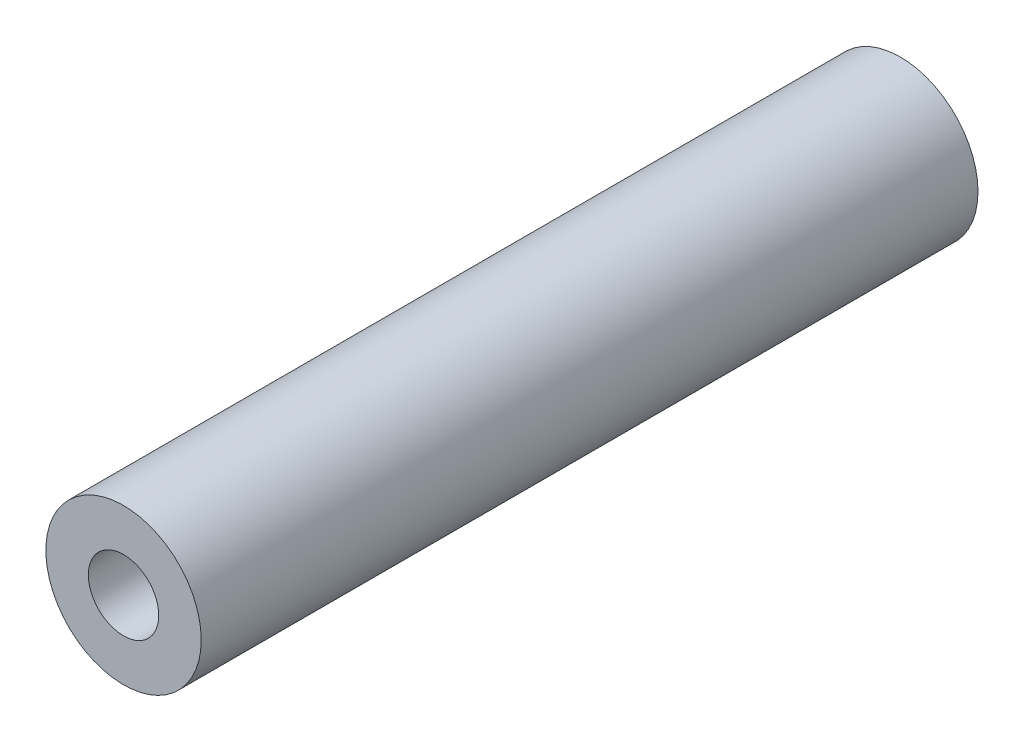
SolidWorks part; units mm, degrees
ref_plane "Front Plane" through (0, 0, 0) normal (0, 0, 1) x (1, 0, 0)
ref_plane "Top Plane" through (0, 0, 0) normal (0, 1, 0) x (1, 0, 0)
ref_plane "Right Plane" through (0, 0, 0) normal (1, 0, 0) x (0, 0, -1)
other "Configuration Table"
sketch "Sketch1" plane through (0, 0, 0) normal (0, 0, 1) x (1, 0, 0)
  circle A0 centre (0, 0) radius 7.5
  dimension "D1" = 15
extrude "Boss-Extrude1" add sketch "Sketch1" along normal blind 75
hole_wizard "M8 Tapped Hole1" positions "Sketch2" profile "Sketch3" tap size "M8" standard "GB"
sketch "Sketch2" plane through (0, 0, 75) normal (0, 0, 1) x (1, 0, 0)
  point P0 (0, 0)
sketch "Sketch3" plane through (0, 0, 75) normal (1, 0, 0) x (0, -1, 0)
  line L0 (0, 0) -> (0, 21.7929)
  line L1 (0, 21.7929) -> (3.4, 19.75)
  line L2 (3.4, 19.75) -> (3.4, 0)
  line L5 (3.4, 0) -> (0, 0)
  line L10 (0, 21.7929) -> (-3.4, 19.75) construction
  line L11 (0, -6.35) -> (0, 107.95) construction
  dimension "螺纹孔钻头直径" = 6.8
  dimension "螺纹孔钻头深度" = 19.75
  dimension "导头角度" = 118
cosmetic thread "Cosmetic Thread1" parameters "D1"=16, "D2"=8
hole_wizard "M8 Tapped Hole2" positions "Sketch4" profile "Sketch5" tap size "M8" standard "GB"
sketch "Sketch4" plane through (0, 0, 0) normal (0, 0, -1) x (-1, 0, 0)
  point P0 (0, 0)
sketch "Sketch5" plane through (0, 0, 0) normal (1, 0, 0) x (0, 1, 0)
  line L0 (0, 0) -> (0, 21.7929)
  line L1 (0, 21.7929) -> (3.4, 19.75)
  line L2 (3.4, 19.75) -> (3.4, 0)
  line L5 (3.4, 0) -> (0, 0)
  line L10 (0, 21.7929) -> (-3.4, 19.75) construction
  line L11 (0, -6.35) -> (0, 107.95) construction
  dimension "螺纹孔钻头直径" = 6.8
  dimension "螺纹孔钻头深度" = 19.75
  dimension "导头角度" = 118
cosmetic thread "Cosmetic Thread2"
